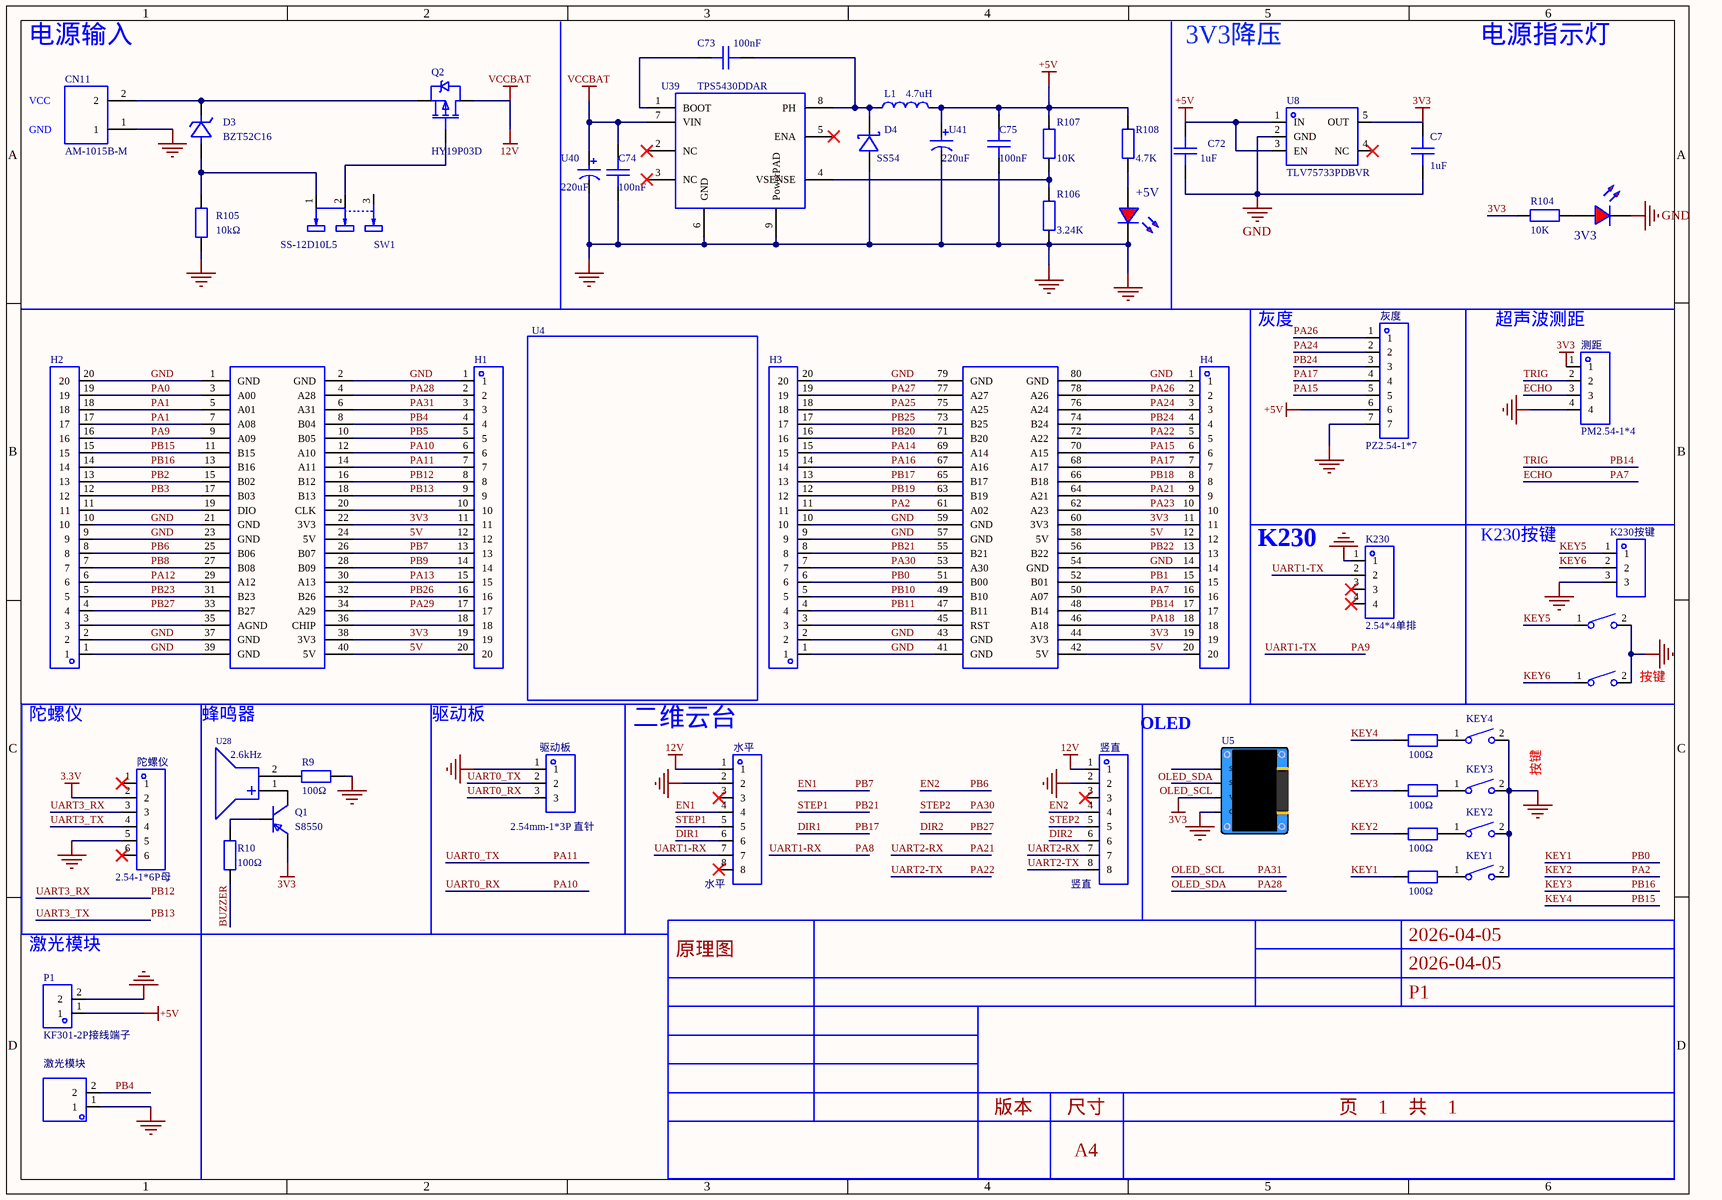
[diagram p0: MISC49913-2.schdoc]
# Altium project MISC49913-3.PrjPcb
1 sheet, 52 parts. Net scope: global (net labels, ports and power ports of the same name join across sheets).
Board file: MISC49913.pcbdoc

## Sheet MISC49913-2.schdoc
size 297 x 209 mm; Version: V1.0; @Project Name: MISC49913; @Page Count: 1; @Update Date: 2026-04-05; @Create Date: 2026-04-05; @Schematic Name: MISC49913; @Page No: 1; @Board Name: MISC49913; @Create Time: 12:57:04; @Update Time: 22:24:49; Size: A4

### Parts
3V3  (no value)  [LED_0603]
+5V  (no value)  [LED_0603]
C7  1uF  [C0603]
C72  1uF  [C0603]
C73  100nF  [C0805]
C74  100nF  [C0805]
C75  100nF  [C0805]
CN11  AM-1015B-M  [CONN-TH_AM-1015B-M]
D3  BZT52C16  [SOD-123_L2.7-W1.6-LS3.7-RD]
D4  SS54  [SMA_L4.4-W2.8-LS5.4-R-RD]
H1  (no value)  [HDR-TH_20P-P2.54-V-M-1]
H2  (no value)  [HDR-TH_20P-P2.54-V-M-1]
H3  (no value)  [HDR-TH_20P-P2.54-V-M-1]
H4  (no value)  [HDR-TH_20P-P2.54-V-M-1]
K230  2.54*4单排  [HDR-TH_4P-P2.54-V-M-1]
K230按键  K230按键  [HDR-TH_3P-P2.54-V-M]
K230按键1  轻触按键3*6*2.5  [SW-SMD_L6.0-W3.6-LS8.0]  (value not drawn)
K230按键2  轻触按键3*6*2.5  [SW-SMD_L6.0-W3.6-LS8.0]  (value not drawn)
KEY1  轻触按键3*6*2.5  [SW-SMD_L6.0-W3.6-LS8.0]  (value not drawn)
KEY2  轻触按键3*6*2.5  [SW-SMD_L6.0-W3.6-LS8.0]  (value not drawn)
KEY3  轻触按键3*6*2.5  [SW-SMD_L6.0-W3.6-LS8.0]  (value not drawn)
KEY4  轻触按键3*6*2.5  [SW-SMD_L6.0-W3.6-LS8.0]  (value not drawn)
L1  4.7uH  [IND-SMD_L7.3-W6.6]
P1  KF301-2P接线端子  [CONN-TH_XY301V-A-5.0-2P]
Q1  S8550  [SOT-23-3_L2.9-W1.6-P1.90-LS2.8-BR]
Q2  HY19P03D  [TO-252-2_L6.6-W6.1-P4.57-LS9.9-TL-CW]
R9  100Ω  [R0603]
R10  100Ω  [R0603]
R104  10K  [R0603]
R105  10kΩ  [R0603]
R106  3.24K  [R0603]
R107  10K  [R0603]
R108  4.7K  [R0603]
R109  100Ω  [R0603]
R110  100Ω  [R0603]
R111  100Ω  [R0603]
R112  100Ω  [R0603]
SW1  SS-12D10L5  [SW-TH_SS-12D10L5]
U4  (no value)  [COMM-TH_LCKFB-TMX-MSPM0G3507]
U5  (no value)  [0.96OLED_4P]
U8  TLV75733PDBVR  [SOT-23-5_L2.9-W1.6-P0.95-LS2.8-BL]
U28  2.6kHz  [BUZ-TH_BD12.0-P7.60-D0.6-FD]
U39  TPS5430DDAR  [ESOP-8_L4.9-W3.9-P1.27-LS6.0-TL-EP]
U40  220uF  [CAP-SMD_BD6.3-L6.6-W6.6-LS7.2-FD]
U41  220uF  [CAP-SMD_BD6.3-L6.6-W6.6-LS7.2-FD]
水平  水平  [CONN-TH_8P-P2.50-XH2.54-8P]
测距  PM2.54-1*4  [HDR-TH_4P-P2.54-V-F]
激光模块  (no value)  [HDR-TH_2P-P2.54-V-M-1]
灰度  PZ2.54-1*7  [HDR-TH_7P-P2.54-V-M]
竖直  竖直  [CONN-TH_8P-P2.50-XH2.54-8P]
陀螺仪  2.54-1*6P母  [HDR-TH_6P-P2.54-V-F]
驱动板  2.54mm-1*3P 直针  [HDR-TH_3P-P2.54-V-M-1]

### Nets
3.3V: 陀螺仪.2
3V3: C7.2 H1.11 H1.19 H4.11 H4.19 Q1.2 R104.1 U4.22(3V3) U4.38(3V3) U4.44(3V3) U4.60(3V3) U5.2(VCC) U8.5(OUT) 测距.1
12V: C74.2 Q2.2(D) U39.7(VIN) U40.1 水平.1 竖直.1  [also labelled VCCBAT]
+5V: C72.2 C75.2 L1.2 P1.1 R107.2 R108.2 U8.1(IN) U8.3(EN) U41.1 灰度.6
GND: 3V3.1(C) +5V.1(C) C7.1 C72.1 C74.1 C75.1 CN11.1 D4.1(A) H1.1 H2.1 H2.2 H2.9 H2.10 H2.20 H3.1 H3.2 H3.9 H3.10 H3.20 H4.1 H4.14 K230.1 K230按键.3 K230按键1.2 K230按键2.2 KEY1.2 KEY2.2 KEY3.2 KEY4.2 P1.2 R9.1 R105.1 R106.1 U4.1(GND) U4.2(GND) U4.21(GND) U4.23(GND) U4.37(GND) U4.39(GND) U4.41(GND) U4.43(GND) U4.54(GND) U4.57(GND) U4.59(GND) U4.79(GND) U4.80(GND) U5.1(GND) U8.2(GND) U39.6(GND) U39.9(PowerPAD) U40.2 U41.2 水平.2 测距.4 激光模块.1 灰度.7 竖直.2 陀螺仪.5 驱动板.1
5V: H1.12 H1.20 H4.12 H4.20 U4.24(5V) U4.40(5V) U4.42(5V) U4.58(5V)
BUZZER: R10.2
DIR1: H3.13 U4.65(B17) 水平.6  [also labelled PB17]
DIR2: H2.4 U4.33(B27) 竖直.6  [also labelled PB27]
ECHO: H4.16 U4.50(A07) 测距.3  [also labelled PA7]
EN1: H1.13 U4.26(B07) 水平.4  [also labelled PB7]
EN2: H2.8 U4.25(B06) 竖直.4  [also labelled PB6]
KEY1: H3.6 R109.2 U4.51(B00)  [also labelled PB0]
KEY2: H3.11 R110.2 U4.61(A02)  [also labelled PA2]
KEY3: H2.14 R111.2 U4.13(B16)  [also labelled PB16]
KEY4: H2.15 R112.2 U4.11(B15)  [also labelled PB15]
KEY5: K230按键.1 K230按键1.1
KEY6: K230按键.2 K230按键2.1
OLED_SCL: H1.3 U4.6(A31) U5.3(SCL)  [also labelled PA31]
OLED_SDA: H1.2 U4.4(A28) U5.4(SDA)  [also labelled PA28]
PA0: H2.19 U4.3(A00)
PA1: H2.17 H2.18 U4.5(A01) U4.7(A08)
PA8: 水平.7  [also labelled UART1-RX]
PA9: H2.16 K230.2 U4.9(A09)  [also labelled UART1-TX]
PA10: H1.6 U4.12(A10) 驱动板.3  [also labelled UART0_RX]
PA11: H1.7 U4.14(A11) 驱动板.2  [also labelled UART0_TX]
PA12: H2.6 U4.29(A12)
PA13: H1.15 U4.30(A13)
PA14: H3.15 U4.69(A14)
PA15: H4.6 U4.70(A15) 灰度.5
PA16: H3.14 U4.67(A16)
PA17: H4.7 U4.68(A17) 灰度.4
PA18: H4.18 U4.46(A18)
PA21: H4.9 U4.64(A21) 竖直.7  [also labelled UART2-RX]
PA22: H4.5 U4.72(A22) 竖直.8  [also labelled UART2-TX]
PA23: H4.10 U4.62(A23)
PA24: H4.3 U4.76(A24) 灰度.2
PA25: H3.18 U4.75(A25)
PA26: H4.2 U4.78(A26) 灰度.1
PA27: H3.19 U4.77(A27)
PA29: H1.17 U4.34(A29)
PA30: H3.7 U4.53(A30) 竖直.5  [also labelled STEP2]
PB1: H4.15 U4.52(B01)
PB2: H2.13 U4.15(B02)
PB3: H2.12 U4.17(B03)
PB4: H1.4 U4.8(B04) 激光模块.2
PB5: H1.5 U4.10(B05)
PB8: H2.7 U4.27(B08)
PB9: H1.14 U4.28(B09)
PB10: H3.5 U4.49(B10)
PB11: H3.4 U4.47(B11)
PB12: H1.8 U4.16(B12) 陀螺仪.3  [also labelled UART3_RX]
PB13: H1.9 U4.18(B13) 陀螺仪.4  [also labelled UART3_TX]
PB14: H4.17 U4.48(B14) 测距.2  [also labelled TRIG]
PB18: H4.8 U4.66(B18)
PB19: H3.12 U4.63(B19)
PB20: H3.16 U4.71(B20)
PB21: H3.8 U4.55(B21) 水平.5  [also labelled STEP1]
PB22: H4.13 U4.56(B22)
PB23: H2.5 U4.31(B23)
PB24: H4.4 U4.74(B24) 灰度.3
PB25: H3.17 U4.73(B25)
PB26: H1.16 U4.32(B26)
Net3V3_2: 3V3.2(A) R104.2
Net+5V_2: +5V.2(A) R108.1
NetC73_1: C73.1 U39.1(BOOT)
NetC73_2: C73.2 D4.2(K) L1.1 U39.8(PH)
NetCN11_2: CN11.2 D3.1(K) Q2.3(S)
NetD3_2: D3.2(A) R105.2 SW1.1
NetH1_10: H1.10 U4.20(CLK)
NetH1_18: H1.18 U4.36(CHIP)
NetH2_3: H2.3 U4.35(AGND)
NetH2_11: H2.11 U4.19(DIO)
NetH3_3: H3.3 U4.45(RST)
NetKEY1_1: KEY1.1 R109.1
NetKEY2_1: KEY2.1 R110.1
NetKEY3_1: KEY3.1 R111.1
NetKEY4_1: KEY4.1 R112.1
NetQ1_1: Q1.1 R10.1
NetQ1_3: Q1.3 U28.1(+)
NetQ2_1: Q2.1(G) SW1.2
NetR9_2: R9.2 U28.2(-)
NetR106_2: R106.2 R107.1 U39.4(VSENSE)

Not connected (* = marked no-connect by the designer): K230 3* 4*; SW1 3; U8 4(NC)*; U39 2(NC)* 3(NC)* 5(ENA)*; 水平 3* 8*; 竖直 3*; 陀螺仪 1* 6*

### Notes on the sheet
- (near CN11) 电源输入
- 3V3降压
- 电源指示灯
- VCC
- GND
- 灰度
- (near 测距) 超声波测距
- K230
- (near H2) 陀螺仪
- 蜂鸣器
- 驱动板
- OLED
- 按键
- 二维云台
- (near P1) 激光模块
- 2026-04-05
- 原理图
- P1
- 版本
- 尺寸
- A4
- 页    1    共    1

### Library data of the parts
3V3 +5V = LED_0603-R: Symbol: LED_R; Convert to PCB: yes; 3D Model: dd8257b0d61a4cd7b68939a056e08095; 3D Model Transform: 58.72,29.4,22.03,0,0,0,0,0,0; ModelName: LED-0603_R; Device: LED_0603-R; Add into BOM: yes; Supplier Footprint: 0603; FootprintName: LED_0603
C7 C72 = CAP_0603: ConvertToPcb: yes; SymbolName: Capacitance; ModelId: ac125912035d415993ca9572d50418b1; ModelName: C0603_L1.6-W0.8-H0.8; ModelTransform: 62.992,31.496,0,0,0,0,0,0,0; Value: 1uF; Device: CAP_0603; AddInBom: yes; Supplier Footprint: 0603; FootprintName: C0603
C73-C75 = CC0805KRX7R9BB104: 容值:100nF;精度:±10%;额定电压:50V;温度系数:X7R;; Manufacturer: YAGEO(国巨); AddInBom: yes; ModelId: 1ba041120af144c991958decab20d241; ModelName: C0805_L2.0-W1.3-H1.3; ModelTransform: 78.74,51.181,0,0,0,0,0,0.0005,0; Tolerance: ±10%; Voltage Rating: 50V; Temperature Coefficient: X7R; Symbol: CC0805KRX7R9BB104; Device: CC0805KRX7R9BB104; LCSC Part Name: 100nF ±10% 50V; SupplierPart: C49678; ManufacturerPart: CC0805KRX7R9BB104; Supplier Footprint: 0805; JLCPCB Part Class: 基础库; Datasheet: https://item.szlcsc.com/datasheet/CC0805KRX7R9BB104/50686.html; Supplier: LCSC; ConvertToPcb: yes; FootprintName: C0805; Value: 100nF
CN11 = AM-1015B-M: 金属材质：铜镀金  绝缘材质：PA; Manufacturer: AMASS(艾迈斯); AddInBom: yes; ModelId: 846fef71626148f19177cc18c54a3e04; ModelTransform: 314.96,523.621,0,270,0,0,9.601,0.82,-177.165; Symbol: AM-1015B-M; Device: AM-1015B-M; LCSC Part Name: AMASS(艾迈斯)电源连接器公头AM-1015B-M; SupplierPart: C90631; ManufacturerPart: AM-1015B-M; Supplier Footprint: -; JLCPCB Part Class: 扩展库; Datasheet: https://item.szlcsc.com/datasheet/AM-1015B-M/91818.html; Supplier: LCSC; ConvertToPcb: yes; FootprintName: CONN-TH_AM-1015B-M; ModelName: CONN-TH_AM-1015B-M
D3 = BZT52C16: 二极管配置:独立式;稳压值(标称值):16V;稳压值(范围):15.3V~17.1V;耗散功率(Pd):500mW;; Manufacturer: Slkor(萨科微); Symbol: BZT52C16_C707145; AddInBom: yes; ModelId: ad7e39f9e5534b3c96ffdc5532ebb493; ModelName: SOD-123_L2.7-W1.6-H1.4-LS3.7; ModelTransform: 146.026,62.992,0,180,0,0,0.0005,0,0; Diode Configuration: 独立式; Zener Voltage(Nom): 16V; Reverse Leakage Current (Ir): 100nA; Pd - Power Dissipation: 500mW; Impedance(Zzt): 40Ω; Operating Junction Temperature Range: -65℃~+150℃; Device: BZT52C16; LCSC Part Name: 独立式 耐压:16V 电流:0.1uA; SupplierPart: C707145; ManufacturerPart: BZT52C16; Supplier Footprint: SOD-123; JLCPCB Part Class: 扩展库; Datasheet: https://item.szlcsc.com/datasheet/BZT52C16/744267.html; Supplier: LCSC; ConvertToPcb: yes; FootprintName: SOD-123_L2.7-W1.6-LS3.7-RD; Zener Voltage(Range): 15.3V~17.1V
D4 = SS54_C22452: 二极管配置:独立式;正向压降(Vf):550mV@5A;直流反向耐压(Vr):40V;整流电流:5A;; Manufacturer: MDD(辰达半导体); AddInBom: yes; ModelId: 228de99b63224bd3982b21290755dd84; ModelTransform: 204.724,110.236,0,0,0,0,0,0,0; Diode Configuration: 独立式; Voltage - DC Reverse(Vr): 40V; Current - Rectified: 5A; Reverse Leakage Current (Ir): 1mA@40V; Operating Junction Temperature Range: -55℃~+125℃; Symbol: SS54_C22452; Device: SS54_C22452; LCSC Part Name: 电压:40V 电流:5A; SupplierPart: C22452; ManufacturerPart: SS54; Supplier Footprint: SMA(DO-214AC); JLCPCB Part Class: 基础库; Datasheet: https://item.szlcsc.com/datasheet/SS54/23178.html; Supplier: LCSC; ConvertToPcb: yes; FootprintName: SMA_L4.4-W2.8-LS5.4-R-RD; ModelName: SMA_L4.4-W2.8-LS5.4-R-RD; Voltage - Forward(Vf@If): 550mV@5A
H1-H4 = HDR-M_2.54_1x20P: 间距:2.54mm;总PIN位数:20;排数:1;插针结构:-;行距:-;安装类型:直插;圆针/方针:-;额定电流:-;额定电压:-;配合针长度:-;塑高:-;触头材质:黄铜;触头镀层:-;颜色:黑色;; Symbol: HDR_2.54-1x20P; ConvertToPcb: yes; ModelId: f68709be121d406db68b06f32a595389; ModelName: HDR-M-2.54_1x20; ModelTransform: 1999.996,100,0,0,0,0,0,2.48,-118.11; Device: HDR-M_2.54_1x20P; AddInBom: yes; SupplierPart: C50981; Supplier Footprint: 插件; FootprintName: HDR-TH_20P-P2.54-V-M-1
K230 = 2.54*4单排: AddInBom: yes; ModelId: e2e03939c192453cba872779c0cb6390; ModelTransform: 400.039,100,0,0,0,0,0,0,-118.11; Symbol: 2.54*4单排; Device: 2.54*4单排; LCSC Part Name: 2.54*4单排; SupplierPart: C9900016163; ManufacturerPart: 2.54*4单排; Supplier Footprint: 2.54x4; JLCPCB Part Class: 扩展库; Supplier: LCSC; ConvertToPcb: yes; FootprintName: HDR-TH_4P-P2.54-V-M-1; ModelName: HDR-TH_4P-P2.54-V-M-1
K230按键 = HDR-M_2.54_1x3P: AddInBom: yes; ModelId: bb473b6d38ff42a99216a4fcdbdcc4cb; ModelName: HDR-TH_3P-P2.54-M-LI-1X3P; ModelTransform: 300.03877,100,0,0,0,0,0,0,-118.11; Device: HDR-M_2.54_1x3P; Symbol: HDR-M_2.54_1x3P; ConvertToPcb: yes; FootprintName: HDR-TH_3P-P2.54-V-M; SupplierPart: C2937625; Supplier Footprint: 插件; JLCPCB Part Class: 扩展库
K230按键1 K230按键2 KEY1-KEY4 = 轻触按键3*6*2.5: AddInBom: yes; ModelId: 5cda64a5897044e48badc24f5aa7d420; ModelName: SW-SMD_L6.0-W3.6-H2.5-LS8.0; ModelTransform: 314.96,141.732,0,0,0,0,0,0,0; Symbol: 轻触按键3*6*2.5; Device: 轻触按键3*6*2.5; LCSC Part Name: 轻触按键3*6*2.5; SupplierPart: C9900013040; ManufacturerPart: 轻触按键3*6*2.5; Supplier Footprint: KEY; JLCPCB Part Class: 扩展库; Supplier: LCSC; ConvertToPcb: yes; FootprintName: SW-SMD_L6.0-W3.6-LS8.0
L1 = MCS0630-4R7MPY1: 电感值:4.7uH;精度:±20%;额定电流:5.5A;饱和电流(Isat):7A;; Manufacturer: PSA(信昌电陶); AddInBom: yes; ModelId: f365aa58eec94c2a8dfc1404764b7425; ModelName: IND-SMD_L7.1-W6.6-H2.8; ModelTransform: 279.527,259.842,0,0,0,0,0.0005,0,0; Tolerance: ±20%; Rated Current: 5.5A; Saturation Current (Isat): 7A; DC Resistance (DCR): 37mΩ; Symbol: MCS0630-4R7MPY1; Device: MCS0630-4R7MPY1; LCSC Part Name: 4.7uH ±20% 7A; SupplierPart: C2937097; ManufacturerPart: MCS0630-4R7MPY1; Supplier Footprint: 0630; JLCPCB Part Class: 扩展库; Datasheet: https://atta.szlcsc.com/upload/public/pdf/source/20220121/EA6E6E6F70ED7BAE67EC293805EAAACB.pdf; Supplier: LCSC; ConvertToPcb: yes; FootprintName: IND-SMD_L7.3-W6.6; Value: 4.7uH
P1 = KF301-2P接线端子: AddInBom: yes; ModelId: ef7ead88b0f2448d904975b26718870f; ModelTransform: 417.322,299.212,0,0,0,0,11.811,-7.835,-157.48; Symbol: KF301-2P接线端子; Device: KF301-2P接线端子; LCSC Part Name: KF301-2P接线端子; SupplierPart: C9900016950; ManufacturerPart: KF301-2P接线端子; Supplier Footprint: CK301-2P; JLCPCB Part Class: 扩展库; Supplier: LCSC; ConvertToPcb: yes; FootprintName: CONN-TH_XY301V-A-5.0-2P; ModelName: CONN-TH_XY301V-A-5.0-2P
Q1 = S8550_C105432: 晶体管类型:PNP;集电极电流(Ic):500mA;集射极击穿电压(Vceo):25V;功率(Pd):300mW;直流电流增益(hFE@Ic,Vce):120@50mA,1V;; Manufacturer: CJ(江苏长电/长晶); AddInBom: yes; ModelId: 89cb27a44ab2466697082bb9fd73a7d0; ModelName: SOT-23-3L_L2.9-W1.6-H1.1-LS2.8-P0.95; ModelTransform: 114.173,110.236,0,90,0,0,0,0,0; Transistor Type: PNP; Collector Current (Ic): 500mA; Collector-Emitter Breakdown Voltage (Vceo): 25V; Power Dissipation (Pd): 300mW; Transition Frequency (fT): 150MHz; Collector Cut-Off Current (Icbo): 100nA; Collector-Emitter Saturation Voltage (VCE(sat)@Ic,Ib): 600mV@500mA,50mA; Symbol: S8550_C105432; Device: S8550_C105432; LCSC Part Name: S8550(RANGE:120-200) L档120-200; SupplierPart: C105432; ManufacturerPart: S8550; Supplier Footprint: SOT-23; JLCPCB Part Class: 基础库; Datasheet: https://atta.szlcsc.com/upload/public/pdf/source/20171228/C164891_15144412930301213894.pdf; Supplier: LCSC; ConvertToPcb: yes; FootprintName: SOT-23-3_L2.9-W1.6-P1.90-LS2.8-BR; DC Current Gain (hFE@Ic,Vce): 120@50mA,1V; Operating Temperature: -
Q2 = HY19P03D: 类型:P沟道;漏源电压(Vdss):30V;连续漏极电流(Id):90A;功率(Pd):50W;导通电阻(RDS(on)@Vgs,Id):6mΩ@10V,45A;阈值电压(Vgs(th)@Id):3V@250uA;; Manufacturer: HUAYI(华羿微); AddInBom: yes; ModelId: ce57f84d66384067af8a68020b6de06d; ModelName: TO-252-2L-3P_L6.6-W6.1-H2.3-LS10.1-P4.6; ModelTransform: 259.842,390.52442,0,270,0,0,38.027,-0.598,0; Type: P沟道; Drain Source Voltage (Vdss): 30V; Continuous Drain Current (Id): 90A; Power Dissipation (Pd): 50W; Symbol: HY19P03D; Device: HY19P03D; LCSC Part Name: P沟道 耐压:30V 电流:90A; SupplierPart: C122492; ManufacturerPart: HY19P03D; Supplier Footprint: TO-252-2; JLCPCB Part Class: 扩展库; Datasheet: https://atta.szlcsc.com/upload/public/pdf/source/20170728/C122492_1501225751911848809.pdf; Supplier: LCSC; ConvertToPcb: yes; FootprintName: TO-252-2_L6.6-W6.1-P4.57-LS9.9-TL-CW; Drain Source On Resistance (RDS(on)@Vgs,Id): 6mΩ@10V,45A; Gate Threshold Voltage (Vgs(th)@Id): 3V@250uA
R9 R10 R104 R106-R108 = Res_0603: Symbol: 电阻; ConvertToPcb: yes; ModelId: fc143cca1e79419f9cd78b61e9279f08; ModelTransform: 31.8897,63.7794,0,90,0,0,0,0,0; Device: Res_0603; AddInBom: yes; Supplier Footprint: 0603; FootprintName: R0603; ModelName: R0603
  R9 R10: Value: 100Ω
  R104 R107: Value: 10K
  R106: Value: 3.24K
  R108: Value: 4.7K
R105 = 0603WAF1002T5E: 电阻类型:厚膜电阻;阻值:10kΩ;精度:±1%;功率:100mW;最大工作电压:75V;温度系数:±100ppm/℃;; Manufacturer: UNI-ROYAL(厚声); AddInBom: yes; ModelId: fc143cca1e79419f9cd78b61e9279f08; ModelTransform: 31.8897,63.7794,0,90,0,0,0,0,0; Tolerance: ±1%; Power(Watts): 100mW; Overload Voltage (Max): 75V; Symbol: 0603WAF1002T5E; Device: 0603WAF1002T5E; Supplier: LCSC; Manufacturer Part: 0603WAF1002T5E; Supplier Part: C25804; Value: 10kΩ; JLCPCB Part Class: 基础库; LCSC Part Name: 厚膜电阻 10kΩ ±1% 100mW; Supplier Footprint: 0603; Datasheet: https://atta.szlcsc.com/upload/public/pdf/source/20200306/C422600_1E6D84923E4A46A82E41ADD87F860B5C.pdf; ConvertToPcb: yes; FootprintName: R0603; ModelName: R0603; Type: 厚膜电阻; Temperature Coefficient: ±100ppm/℃; Operating Temperature Range: -55℃~+155℃
R109-R112 = 0603WAF1000T5E: 电阻类型:厚膜电阻;阻值:100Ω;精度:±1%;功率:100mW;最大工作电压:75V;温度系数:±200ppm/℃;; Manufacturer: UNI-ROYAL(厚声); AddInBom: yes; ModelId: fc143cca1e79419f9cd78b61e9279f08; ModelTransform: 31.8897,63.7794,0,90,0,0,0,0,0; Tolerance: ±1%; Power(Watts): 100mW; Overload Voltage (Max): 75V; Symbol: 0603WAF1000T5E; Device: 0603WAF1000T5E; LCSC Part Name: 100Ω ±1% 100mW 厚膜电阻; SupplierPart: C22775; ManufacturerPart: 0603WAF1000T5E; Supplier Footprint: 0603; JLCPCB Part Class: 基础库; Datasheet: https://atta.szlcsc.com/upload/public/pdf/source/20200306/C422600_1E6D84923E4A46A82E41ADD87F860B5C.pdf; Supplier: LCSC; ConvertToPcb: yes; FootprintName: R0603; ModelName: R0603; Type: 厚膜电阻; Value: 100Ω; Temperature Coefficient: ±200ppm/℃; Operating Temperature Range: -55℃~+155℃
SW1 = SS-12D10L5: 电路结构:单刀双掷;安装方式:直插;开关颜色:黑色;额定电流(DC):3A;额定电压(DC):125V;额定电流(AC):3A;额定电压(AC):125V;机械寿命:1万次;; Manufacturer: XKB Connectivity(中国星坤); AddInBom: yes; ModelId: c49f07a32c154ec8ad7cf47670a53981; ModelName: SW-TH_L13.0-W6.8-H6.4-P4.7; ModelTransform: 511.81,267.716,0,0,0,0,0,0,-275.591; Circuit: 单刀双掷; Actuator Style: 矩形柱状; Pin Style: PC引脚; Switch Length: 13mm; Switch Width: 6.8mm; Switch Height: 6.4mm; Actuator Color: 黑色; Current Rating (DC): 3A; Voltage Rating (DC): 125V; Mechanical Life: 1万次; Symbol: SS-12D10L5; Device: SS-12D10L5; LCSC Part Name: 柄长5mm 直插双档 滑动开关; SupplierPart: C319012; ManufacturerPart: SS-12D10L5; Supplier Footprint: 插件; JLCPCB Part Class: 扩展库; Datasheet: https://atta.szlcsc.com/upload/public/pdf/source/20211009/D6412F37AABE6F9459A6EE7FA4DAEADB.pdf; Supplier: LCSC; ConvertToPcb: yes; FootprintName: SW-TH_SS-12D10L5; Mounting Style: 直插; Current Rating (AC): 3A; Voltage Rating (AC): 125V; Operating Temperature: -40℃~+85℃
U4 = LCKFB-TMX-MSPM0G3507: Manufacturer: 立创开发板; AddInBom: yes; ModelId: 8c2b7ba131d4412eae9a4354ab816d50; ModelTransform: 1769.654,2753.608,0,0,0,0,0,-56.102,-236.22; LCSC Part Name: 立创·天猛星MSPM0G3507开发板 5件套; Symbol: LCKFB-TMX-MSPM0G3507; Device: LCKFB-TMX-MSPM0G3507; SupplierPart: C42378531; ManufacturerPart: LCKFB-TMX-MSPM0G3507; Supplier Footprint: -; Datasheet: https://atta.szlcsc.com/upload/public/pdf/source/20241209/800332349277522348D9357AB5109808.pdf; Supplier: LCSC; ConvertToPcb: yes; FootprintName: COMM-TH_LCKFB-TMX-MSPM0G3507; ModelName: COMM-TH_LCKFB-TMX-MSPM0G3507
U5 = 0.96OLED模块_4P: ConvertToPcb: yes; ModelId: 79c000fdb68d45a296c2e9bedf4f9055; ModelTransform: 1393.69792,1318.895,0,0,0,0,0,-560.079,-137.795; Device: 0.96OLED模块_4P; AddInBom: yes; SymbolName: 0.96OLED模块_4P; FootprintName: 0.96OLED_4P; Supplier Footprint: 插件; ModelName: 0.96OLED_4P
U8 = TLV75733PDBVR: 输出类型:固定;最大输入电压:5.5V;输出电压:3.3V;输出电流:1A;电源纹波抑制比(PSRR):52dB;输出极性:正极;; Manufacturer: TI(德州仪器); AddInBom: yes; ModelId: 018c57e721114987ae90467fe9f1d259; ModelTransform: 114.96,110.236,0,0,0,0,0,0,0; Output Type: 固定; Maximum Input Voltage: 5.5V; Output Voltage: 3.3V; Output Current: 1A; Power Supply Rejection Ratio (PSRR): 52dB; Dropout Voltage: 475mV@(1A); Output Polarity: 正极; Number of Outputs: 1; Symbol: TLV75733PDBVR; Device: TLV75733PDBVR; LCSC Part Name: 具有使能功能的 1A、低 IQ、高精度、低压降稳压器; SupplierPart: C485517; ManufacturerPart: TLV75733PDBVR; Supplier Footprint: SOT-23-5; JLCPCB Part Class: 扩展库; Datasheet: https://www.ti.com/cn/lit/gpn/tlv757p; Supplier: LCSC; ConvertToPcb: yes; FootprintName: SOT-23-5_L2.9-W1.6-P0.95-LS2.8-BL; ModelName: SOT-23-5_L2.9-W1.6-P0.95-LS2.8-BL; Feature: 防静电保护；浪涌保护；低ESR；热保护(TSD)；欠压闭锁；过流保护(OCP)；带使能; Operating Temperature: -40℃~+125℃@(Tj)
U28 = HYE1206-05ST: 频率:2.6kHz;声压(SPL):80dB@5V,10cm;; Manufacturer: HYDZ(华宇); AddInBom: yes; ModelId: 16ab50e14c5b4f2c986c135bdba60e37; ModelName: BUZ-TH_D12.0-H9.5-P7.60; ModelTransform: 472.44,472.176,0,90,0,0,-0.787,0,-177.165; Symbol: HYE1206-05ST; Device: HYE1206-05ST; Supplier: LCSC; Supplier Part: C17701079; Manufacturer Part: HYE1206-05ST; LCSC Part Name: 有源蜂鸣器HYE1206-05ST; Supplier Footprint: 插件,D=7.6mm; Datasheet: https://atta.szlcsc.com/upload/public/pdf/source/20230912/EF3443D3A1B92F495A3EE65EE7F2091F.pdf; ConvertToPcb: yes; FootprintName: BUZ-TH_BD12.0-P7.60-D0.6-FD; Value: 2.6kHz; Sound Pressure Level (SPL): 80dB@5V,10cm
U39 = TPS5430DDAR: 功能类型:降压型;输出类型:可调;输入电压:5.5V~36V;输出电压:1.221V~32.04V;输出电流(最大值):3A;; Manufacturer: TI(德州仪器); AddInBom: yes; ModelId: 821ddb58f3244ffb9a5d6f8174c5b14e; ModelTransform: 236.22,192.913,0,0,0,0,0,0,0; Function: 降压型; Output Type: 可调; Output Current (Max): 3A; Switching Frequency: 500kHz; Synchronous Rectification: 否; Number of Outputs: 1; Topology: 降压式; Switch tube (built-in/external): 内置; Symbol: TPS5430DDAR; Device: TPS5430DDAR; LCSC Part Name: 降压 3A 36V; SupplierPart: C9864; ManufacturerPart: TPS5430DDAR; Supplier Footprint: SOIC-8-EP; JLCPCB Part Class: 基础库; Datasheet: https://www.ti.com/cn/lit/gpn/tps5430; Supplier: LCSC; ConvertToPcb: yes; FootprintName: ESOP-8_L4.9-W3.9-P1.27-LS6.0-TL-EP; ModelName: ESOP-8_L4.9-W3.9-P1.27-LS6.0-TL-EP; Input Voltage: 5.5V~36V; Output Voltage: 1.221V~32.04V; Operating Temperature: -40℃~+125℃@(TJ)
U40 U41 = 220uF: AddInBom: yes; ModelId: 1f98774f34d342b59c9890c435f425a3; ModelTransform: 283.464,259.842,0,180,0,0,0,0,0; Symbol: 220UF; Device: 220uF; LCSC Part Name: 220uF; SupplierPart: C2941234; ManufacturerPart: 220uF; Supplier Footprint: -SMD6.3/5.8; JLCPCB Part Class: 扩展库; Supplier: LCSC; ConvertToPcb: yes; FootprintName: CAP-SMD_BD6.3-L6.6-W6.6-LS7.2-FD; ModelName: CAP-SMD_BD6.3-L6.6-W6.6-LS7.2-FD
水平 竖直 = XH2.54-8P 直插: AddInBom: yes; ModelId: 385b1d4b778b4141959d674ea048df76; ModelTransform: 885.825,228.346,0,180,0,0,0.591,-19.094,-137.795; Symbol: XH2.54-8P 直插; Device: XH2.54-8P 直插; LCSC Part Name: XH2.54-8P 直插; SupplierPart: C9900000730; Supplier Footprint: TH-8_5.8X22.5X2.54P; JLCPCB Part Class: 扩展库; Supplier: LCSC; ConvertToPcb: yes; FootprintName: CONN-TH_8P-P2.50-XH2.54-8P; ModelName: CONN-TH_8P-P2.50-XH2.54-8P
  水平: Manufacturer Part: 水平
  竖直: Manufacturer Part: 竖直
测距 = PM2.54-1*4: 插孔结构:1x4P;间距:2.54mm;行距:2.54mm;圆孔/方孔:方孔;安装方式:直插;排数:单排;总孔位数:4P;额定电流:2.5A;插孔方向:顶部;塑高:8.5mm;工作温度:-40℃~+105℃;; Manufacturer: ZHOURI(洲日); AddInBom: yes; ModelId: d187812051054f85879fcaa51a310d8e; ModelTransform: 419.6842,98.464,0,0,0,0,0,0,-118.11; Holes Structure: 1x4P; Pitch: 2.54mm; Circular Hole / Square Hole: 方孔; Number of Positions: 4P; Current Rating: 2.5A; Holes Direction: 顶部; Symbol: PM2.54-1*4; Device: PM2.54-1*4; LCSC Part Name: 间距:2.54mm 1x4P 直插; SupplierPart: C5116530; ManufacturerPart: PM2.54-1*4; Supplier Footprint: 插件,P=2.54mm; JLCPCB Part Class: 扩展库; Datasheet: https://item.szlcsc.com/datasheet/PM2.54-1*4/5692947.html; Supplier: LCSC; ConvertToPcb: yes; FootprintName: HDR-TH_4P-P2.54-V-F; ModelName: HDR-TH_4P-P2.54-V-F; Row Spacing: 2.54mm; Mounting Type: 直插; Number of Rows: 单排; Insulation Height: 8.5mm; Operating Temperature: -40℃~+105℃
激光模块 = HDR-M_2.54_1x2P: Symbol: 210S-1*2P L=11.6MMGold-plated black; ConvertToPcb: yes; ModelId: 79b2e9f2d70a4d68a1b7098f27c6d4c5; ModelName: HDR-M-2.54_1x2; ModelTransform: 200,100,0,0,0,0,0,0,-118.11; Device: HDR-M_2.54_1x2P; AddInBom: yes; SupplierPart: C124375; Supplier Footprint: 插件; FootprintName: HDR-TH_2P-P2.54-V-M-1; JLCPCB Part Class: 扩展库
灰度 = PZ2.54-1*7: 插针结构:1x7P;间距:2.54mm;圆针/方针:方针;安装方式:直插;排数:单排;总PIN位数:7P;额定电流:2.5A;配合针长度:6mm;塑高:2.54mm;端接针长度:3mm;触头材质:黄铜;触头镀层:金;工作温度:-40℃~+105℃;; Manufacturer: ZHOURI(洲日); AddInBom: yes; ModelId: 3f496cdc752348c6a5e9157bbaceaf96; ModelName: HDR-TH_7P-P2.54-M-LI-1X7P; ModelTransform: 690.1561,98.425,0,0,0,0,0,0,-118.11; Pin Structure: 1x7P; Pitch: 2.54mm; Circluar Pins/Square Pins: 方针; Current Rating: 2.5A; Symbol: PZ2.54-1*7; Device: PZ2.54-1*7; LCSC Part Name: 1x7P 间距:2.54mm 方针 直插; SupplierPart: C5360900; ManufacturerPart: PZ2.54-1*7; Supplier Footprint: 插件,P=2.54mm; JLCPCB Part Class: 扩展库; Datasheet: https://item.szlcsc.com/datasheet/PZ2.54-1*7/6180459.html; Supplier: LCSC; ConvertToPcb: yes; FootprintName: HDR-TH_7P-P2.54-V-M; Mounting Type: 直插; Number of Rows: 单排; Number of Pins: 7P; Length of Mating Pin: 6mm; Insulation Height: 2.54mm; Length of End Connection Pin: 3mm; Contact Material: 黄铜; Contact Plating: 金; Operating Temperature: -40℃~+105℃
陀螺仪 = 2.54-1*6P母: 插孔结构:1x6P;间距:2.54mm;行距:-;圆孔/方孔:方孔;安装方式:直插;排数:单排;总孔位数:6P;额定电流:3A;额定电压:-;插孔方向:顶部;塑高:-;触头材质:黄铜;触头镀层:-;工作温度:-40℃~+105℃;; Manufacturer: BOOMELE(博穆精密); Symbol: Header-Female-2.54_1x6; AddInBom: yes; ModelId: 0f5bcf94dcda47d085f24cdca1696fe9; ModelTransform: 619.684,94.488,0,0,0,0,0,0,-125.984; Holes Structure: 1x6P; Pitch: 2.54mm; Circular Hole / Square Hole: 方孔; Number of Positions: 6P; Current Rating: 3A; Holes Direction: 顶部; PIN Length: 3.3mm; Device: 2.54-1*6P母; LCSC Part Name: 1x6P 间距:2.54mm 直插; SupplierPart: C40877; ManufacturerPart: 2.54-1*6P母; Supplier Footprint: 插件,P=2.54mm; JLCPCB Part Class: 扩展库; Datasheet: https://item.szlcsc.com/datasheet/2.54-1*6P%25E6%25AF%258D/41861.html; Supplier: LCSC; ConvertToPcb: yes; FootprintName: HDR-TH_6P-P2.54-V-F; ModelName: HDR-TH_6P-P2.54-V-F; Row Spacing: -; Mounting Type: 直插; Number of Rows: 单排; Voltage Rating (Max): -; Insulation Height: -; Contact Material: 黄铜; Contact Plating: -; Operating Temperature: -40℃~+105℃; Supplementary Features: -
驱动板 = 2.54mm-1*3P 直针: AddInBom: yes; ModelId: 94a8ffe137b6410295cb18cd3ffd99db; ModelName: HDR-M-2.54_1x3; ModelTransform: 299.9994,100,0,0,0,0,0,0,-118.11; Symbol: 2.54MM-1*3P 直针; Device: 2.54mm-1*3P 直针; LCSC Part Name: 2.54mm-1*3P 直针; SupplierPart: C9900025313; ManufacturerPart: 2.54mm-1*3P 直针; Supplier Footprint: 2.54-180-3P; JLCPCB Part Class: 扩展库; Supplier: LCSC; ConvertToPcb: yes; FootprintName: HDR-TH_3P-P2.54-V-M-1